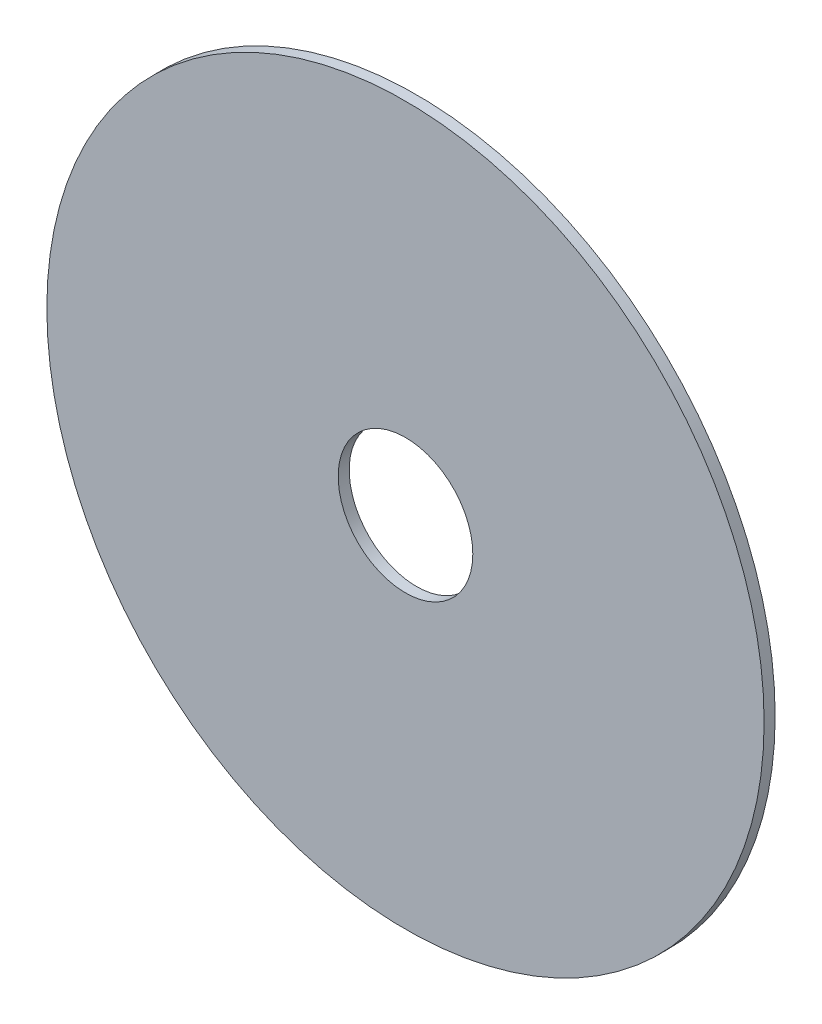
SolidWorks part; units mm, degrees
material "普通碳钢"
ref_plane "Front Plane" through (0, 0, 0) normal (0, 0, 1) x (1, 0, 0)
ref_plane "Top Plane" through (0, 0, 0) normal (0, 1, 0) x (1, 0, 0)
ref_plane "Right Plane" through (0, 0, 0) normal (1, 0, 0) x (0, 0, -1)
sketch "Sketch1" plane through (0, 0, 0) normal (0, 0, 1) x (1, 0, 0)
  circle A0 centre (0, 0) radius 30.5
  circle A1 centre (0, 0) radius 162.5
  dimension "D1" = 325
  dimension "D2" = 61
extrude "Boss-Extrude1" add sketch "Sketch1" along normal blind 5
